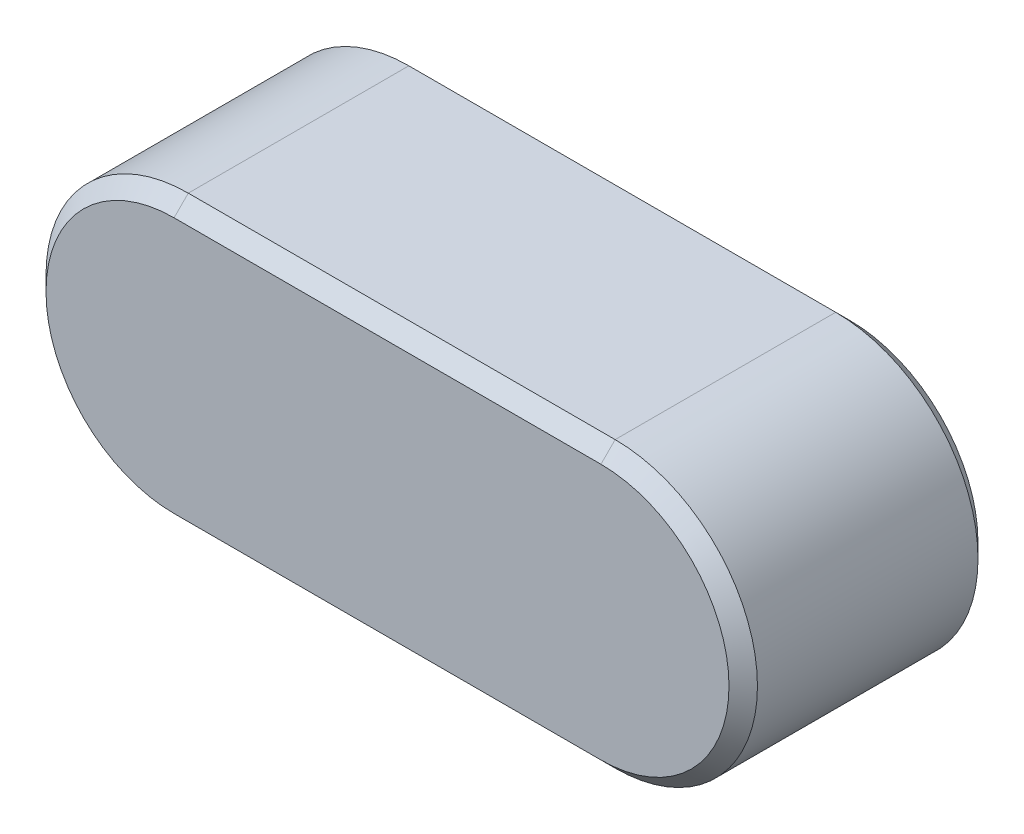
from build123d import *

# Parameters (mm, degrees)
BASEKEY_DEPTH = 3.5
CHAMFER1_SIZE = 0.4


with BuildPart() as part:
    # Sketch1 → BaseKey (new, symmetric)
    with BuildSketch(Plane.XY):
        with BuildLine():
            Line((-12, 4), (0, 4))
            ThreePointArc((0, 4), (4, 0), (0, -4))
            Line((0, -4), (-12, -4))
            ThreePointArc((-12, -4), (-16, 0), (-12, 4))
        make_face()
    extrude(amount=BASEKEY_DEPTH, both=True)

    # Chamfer1
    chamfer1_edges = [part.edges().sort_by_distance(p)[0] for p in [
        (4, 0, 3.5),
        (-6, 4, 3.5),
        (-16, 0, 3.5),
        (-6, 4, -3.5),
        (4, 0, -3.5),
        (-6, -4, -3.5),
        (-16, 0, -3.5),
        (-6, -4, 3.5),
    ]]
    chamfer(chamfer1_edges, length=CHAMFER1_SIZE)


solid = part.part
